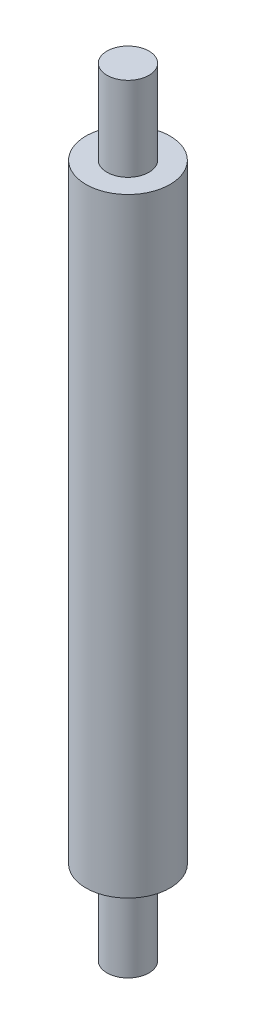
SolidWorks part; units mm, degrees
ref_plane "Front Plane" through (0, 0, 0) normal (0, 0, 1) x (1, 0, 0)
ref_plane "Top Plane" through (0, 0, 0) normal (0, 1, 0) x (1, 0, 0)
ref_plane "Right Plane" through (0, 0, 0) normal (1, 0, 0) x (0, 0, -1)
sketch "Sketch1" plane through (0, 0, 0) normal (1, 0, 0) x (0, 0, -1)
  line L0 (0, 189.9298) -> (0, -191.0006) construction
  line L1 (0, 185) -> (-10, 185)
  line L2 (-10, 185) -> (-10, 145)
  line L3 (-10, 145) -> (-20, 145)
  line L4 (-20, 145) -> (-20, -145)
  line L5 (-20, -145) -> (-10, -145)
  line L6 (-10, -145) -> (-10, -185)
  line L7 (-10, -185) -> (0, -185)
  line L8 (-62.7016, 0) -> (75.2789, 0) construction
  line L9 (0, 185) -> (0, -185)
  dimension "D1" = 290
  dimension "D2" = 10
  dimension "D3" = 20
  dimension "D4" = 40
revolve "Revolve1" add sketch "Sketch1" angle 360 about L0
ref_plane "Plane1" through (0, 0, -10) normal (0, 0, -1) x (-1, 0, 0)
sketch "Sketch2" plane through (0, 0, -10) normal (0, 0, -1) x (-1, 0, 0)
  line L0 (0, 154.7138) -> (0, 101.824) construction
  line L1 (0, 175) -> (0, 155) construction
  line L2 (2.5, 175) -> (2.5, 155)
  line L3 (-2.5, 175) -> (-2.5, 155)
  line L4 (10, 185) -> (-10, 185) construction
  arc A0 (2.5, 175) -> (-2.5, 175) centre (0, 175) ccw
  arc A1 (-2.5, 155) -> (2.5, 155) centre (0, 155) ccw
  point P5 (0, 165)
  dimension "D2" = 2.5
  dimension "D1" = 20
  dimension "D3" = 20
extrude "Cut-Extrude1" cut sketch "Sketch2" against normal blind 2.5
mirror "Mirror1" about plane through (0, 0, 0) normal (0, 1, 0) of "Cut-Extrude1"
